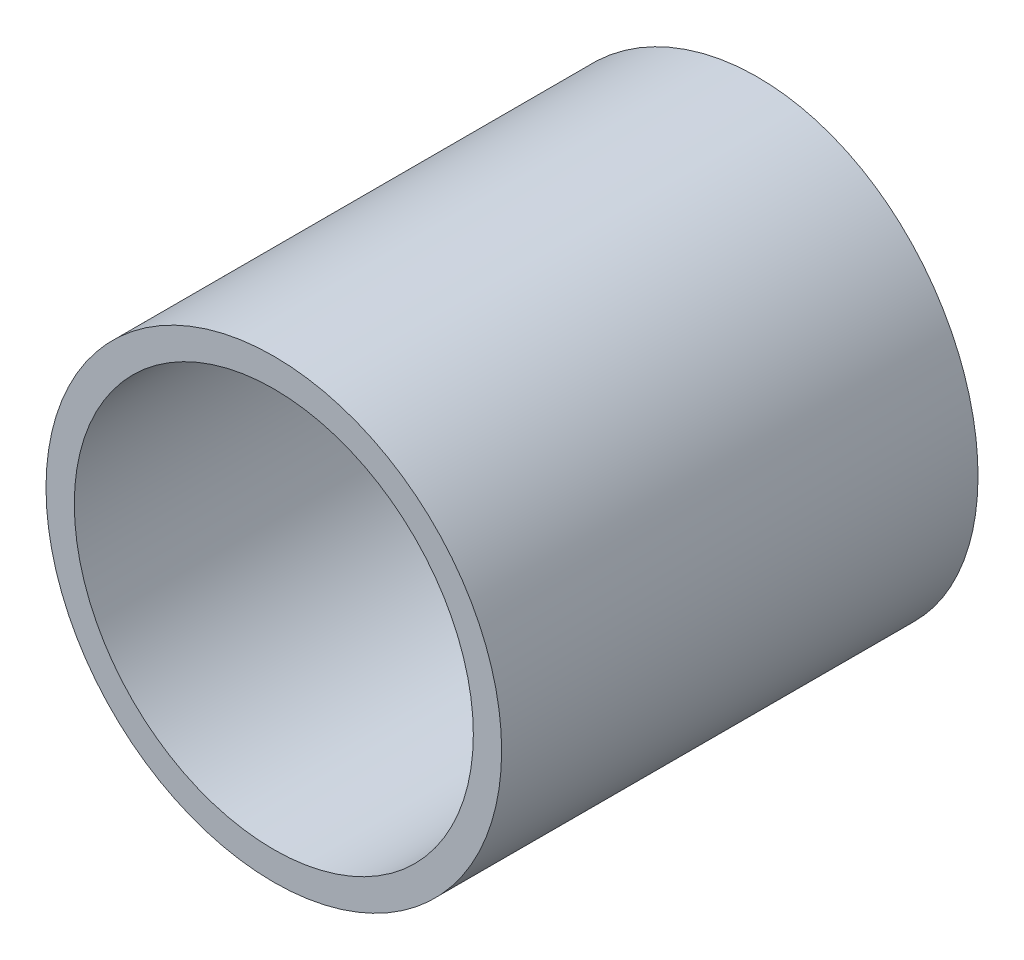
SolidWorks part; units mm, degrees
material "钢管48×4.5/20"
ref_plane "Front Plane" through (0, 0, 0) normal (0, 0, 1) x (1, 0, 0)
ref_plane "Top Plane" through (0, 0, 0) normal (0, 1, 0) x (1, 0, 0)
ref_plane "Right Plane" through (0, 0, 0) normal (1, 0, 0) x (0, 0, -1)
sketch "Sketch1" plane through (0, 0, 0) normal (0, 0, 1) x (1, 0, 0)
  circle A0 centre (0, 0) radius 24.15
  circle A1 centre (0, 0) radius 21.15
  dimension "D1" = 48.3
  dimension "D2" = 3
extrude "Boss-Extrude1" add sketch "Sketch1" along normal blind 100
cosmetic thread "Cosmetic Thread1" parameters "D1"=30, "D2"=44.8
sketch "Sketch3" plane through (0, 0, 0) normal (1, 0, 0) x (0, 0, -1)
  line L0 (0, 0) -> (330, 0) construction
  circle A0 centre (330, 0) radius 379.5
  dimension "D2" = 759
  dimension "D1" = 330
extrude "Cut-Extrude2" cut sketch "Sketch3" against normal mid plane 100 contours A0
